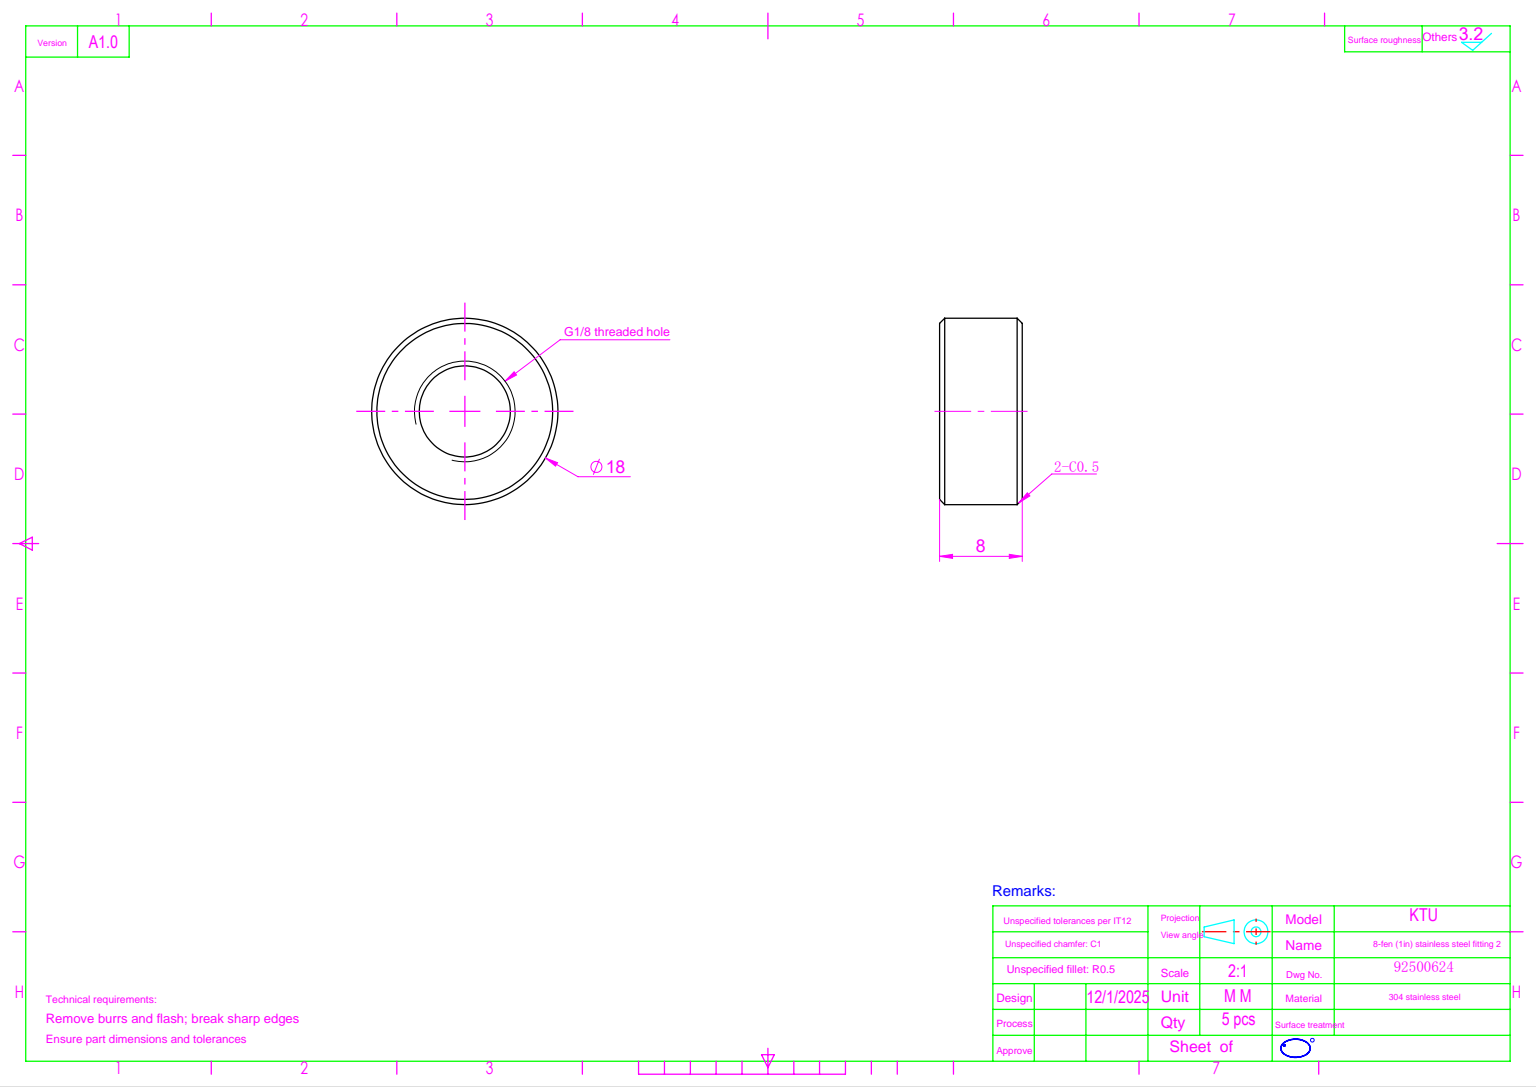
SolidWorks part; units mm, degrees
ref_plane "前视基准面" through (0, 0, 0) normal (0, 0, 1) x (1, 0, 0)
ref_plane "上视基准面" through (0, 0, 0) normal (0, 1, 0) x (1, 0, 0)
ref_plane "右视基准面" through (0, 0, 0) normal (1, 0, 0) x (0, 0, -1)
sketch "草图1" plane through (0, 0, 0) normal (0, 0, 1) x (1, 0, 0)
  circle A0 centre (0, 0) radius 9
  dimension "D1" = 18
extrude "凸台-拉伸1" add sketch "草图1" along normal blind 8
hole_wizard "G1/8 螺纹孔1" positions "草图2" profile "草图3" tap size "G1/8" standard "GB" end condition through all
sketch "草图2" plane through (0, 0, 8) normal (0, 0, 1) x (1, 0, 0)
  point P0 (0, 0)
sketch "草图3" plane through (0, 0, 8) normal (1, 0, 0) x (0, -1, 0)
  line L0 (0, 0) -> (0, 8)
  line L1 (0, 8) -> (4.4, 8)
  line L2 (4.4, 8) -> (4.4, 0)
  line L5 (4.4, 0) -> (0, 0)
  line L11 (0, -6.35) -> (0, 107.95) construction
  dimension "通孔螺纹孔钻头直径" = 8.8
  dimension "通孔螺纹孔钻头深度" = 8
cosmetic thread "孔螺蚊线1" parameters "D2"=9.728
chamfer "倒角1" distance 0.5 angle 45 2 edges at (9, 0, 0) (9, 0, 8)
